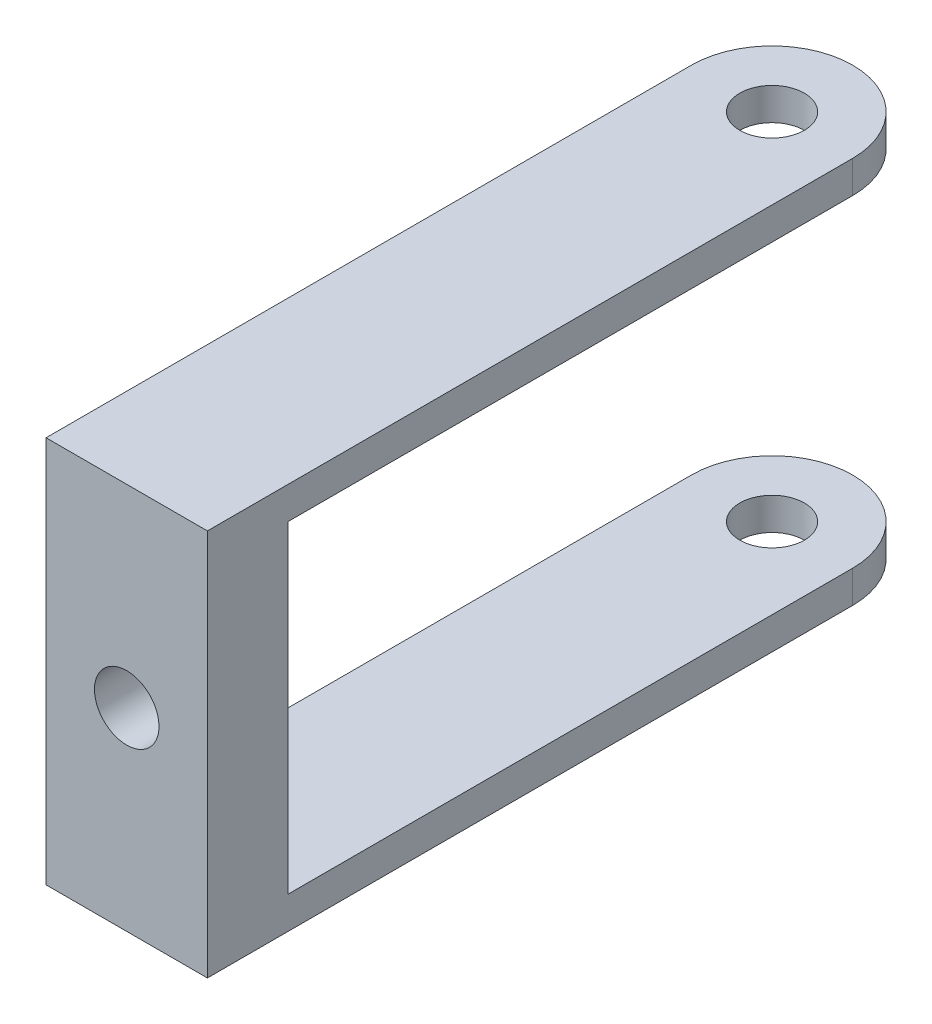
from build123d import *

# Parameters (mm, degrees)
BOSS_EXTRUDE1_DEPTH     = 24
CUT_EXTRUDE1_DEPTH      = 47.914816423
CUT_EXTRUDE1_DEPTH_BACK = 47.914816423
SKETCH2_R               = 2
SKETCH3_W               = 40
SKETCH3_H               = 20
CUT_EXTRUDE2_DEPTH      = 48.707441768
SKETCH4_R               = 2
CUT_EXTRUDE3_DEPTH      = 47.914816423


with BuildPart() as part:
    # Sketch1 → Boss-Extrude1 (new body)
    with BuildSketch(Plane(origin=(0, 0, 0), x_dir=(1, 0, 0), z_dir=(0, 1, 0))):
        with BuildLine():
            Line((-5, 0), (-5, -40))
            Line((-5, -40), (5, -40))
            Line((5, -40), (5, 0))
            ThreePointArc((5, 0), (0, 5), (-5, 0))
        make_face()
    extrude(amount=BOSS_EXTRUDE1_DEPTH)

    # Sketch2 → Cut-Extrude1 (cut, two sides: drawn at the far end of the back side and taken through both)
    with BuildSketch(Plane(origin=(0, 24, 0), x_dir=(1, 0, 0), z_dir=(0, 1, 0)).offset(-CUT_EXTRUDE1_DEPTH_BACK)):
        with Locations(Location((0, 0, 0), (0, 0, 270))):
            Circle(SKETCH2_R)
    extrude(amount=CUT_EXTRUDE1_DEPTH + CUT_EXTRUDE1_DEPTH_BACK, mode=Mode.SUBTRACT)

    # Sketch3 → Cut-Extrude2 (cut, through all)
    with BuildSketch(Plane(origin=(5, 0, 0), x_dir=(0, 0, -1), z_dir=(1, 0, 0))):
        with Locations((-15, 12)):
            Rectangle(SKETCH3_W, SKETCH3_H)
    extrude(amount=-CUT_EXTRUDE2_DEPTH, mode=Mode.SUBTRACT)

    # Sketch4 → Cut-Extrude3 (cut, through all)
    with BuildSketch(Plane(origin=(0, 0, 35), x_dir=(-1, 0, 0), z_dir=(0, 0, -1))):
        with Locations((0, 12)):
            Circle(SKETCH4_R)
    extrude(amount=-CUT_EXTRUDE3_DEPTH, mode=Mode.SUBTRACT)


solid = part.part
